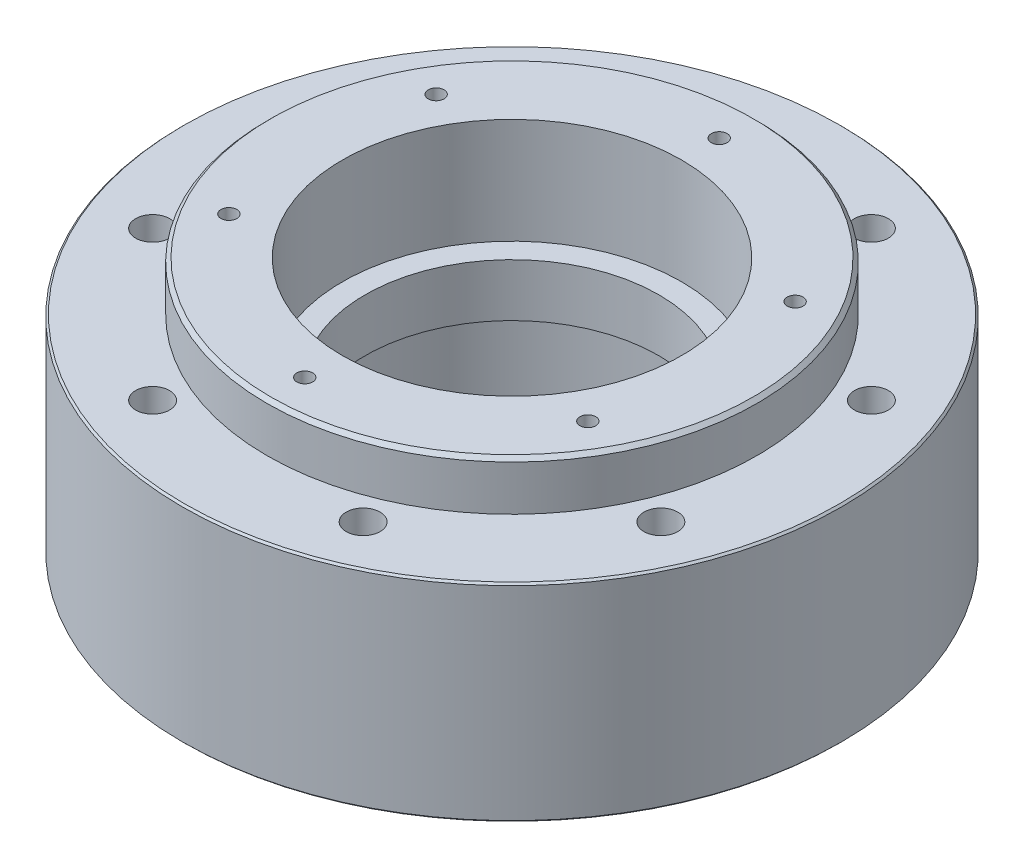
SolidWorks part; units mm, degrees
material "普通碳钢"
ref_plane "Front Plane" through (0, 0, 0) normal (0, 0, 1) x (1, 0, 0)
ref_plane "Top Plane" through (0, 0, 0) normal (0, 1, 0) x (1, 0, 0)
ref_plane "Right Plane" through (0, 0, 0) normal (1, 0, 0) x (0, 0, -1)
sketch "Sketch1" plane through (0, 0, 0) normal (0, 1, 0) x (1, 0, 0)
  circle A0 centre (0, 0) radius 87.5
  dimension "D1" = 175
extrude "Boss-Extrude1" add sketch "Sketch1" along normal blind 55
sketch "Sketch2" plane through (0, 55, 0) normal (0, 1, 0) x (1, 0, 0)
  circle A0 centre (0, 0) radius 65
  dimension "D1" = 130
extrude "Boss-Extrude2" add sketch "Sketch2" along normal blind 13
sketch "Sketch3" plane through (0, 0, 0) normal (0, -1, 0) x (1, 0, 0)
  circle A0 centre (0, 0) radius 57.5
  dimension "D1" = 115
extrude "Boss-Extrude3" add sketch "Sketch3" along normal blind 5
sketch "Sketch4" plane through (0, -5, 0) normal (0, -1, 0) x (1, 0, 0)
  circle A0 centre (0, 0) radius 45
  dimension "D1" = 90
extrude "Cut-Extrude1" cut sketch "Sketch4" against normal blind 31
sketch "Sketch5" plane through (0, 68, 0) normal (0, 1, 0) x (1, 0, 0)
  circle A0 centre (0, 0) radius 45
  dimension "D1" = 90
extrude "Cut-Extrude2" cut sketch "Sketch5" against normal blind 28
sketch "Sketch6" plane through (0, 40, 0) normal (0, 1, 0) x (1, 0, 0)
  circle A0 centre (0, 0) radius 39
  dimension "D1" = 78
extrude "Cut-Extrude3" cut sketch "Sketch6" against normal through all
chamfer "Chamfer1" distance 1 angle 45 2 edges at (0, 68, 65) (0, -5, -57.5)
hole_wizard "Hole size (% based on socket head cap screw type)1" positions "Sketch8" profile "Sketch7" counterbore size "M8" standard "GB" end condition through all
sketch "Sketch8" plane through (0, 0, 0) normal (0, -1, 0) x (-1, 0, 0)
  line L0 (0, 0) -> (0, 104.7926) construction
  line L2 (0, 0) -> (-67.4432, 27.9359) construction
  point P13 (-67.4432, 27.9359)
  dimension "D3" = 67.5
  dimension "D4" = 73
sketch "Sketch7" plane through (67.4432, 0, -27.9359) normal (1, 0, 0) x (0, 0, -1)
  line L0 (0, 0) -> (0, 68)
  line L1 (0, 68) -> (4.5, 68)
  line L3 (4.5, 68) -> (4.5, 30)
  line L4 (4.5, 30) -> (7.5, 30)
  line L5 (7.5, 30) -> (7.5, 0)
  line L7 (7.5, 0) -> (0, 0)
  line L11 (0, -6.35) -> (0, 107.95) construction
  dimension "通孔孔直径" = 9
  dimension "通孔孔深度" = 68
  dimension "柱形沉头孔直径" = 15
  dimension "柱形沉头孔深度" = 30
pattern_circular "CirPattern1" count 8 over 360 about axis through (0, 0, 0) along (0, 1, 0) of "Hole size (% based on socket head cap screw type)1"
chamfer "Chamfer2" distance 0.5 angle 45 2 edges at (0, 55, 87.5) (0, 0, 87.5)
sketch "Sketch12" plane through (0, 68, 0) normal (0, 1, 0) x (1, 0, 0)
  circle A0 centre (0, -50) radius 2.5
  circle A1 centre (0, 0) radius 39 construction
  dimension "D2" = 0
  dimension "D3" = 5
  dimension "D1" = 50
extrude "Cut-Extrude7" cut sketch "Sketch12" against normal blind 22.5
cosmetic thread "Cosmetic Thread2" [suppressed] parameters "D1"=10, "D2"=6
hole_wizard "M10 Tapped Hole1" positions "Sketch14" profile "Sketch13" tap size "M10" standard "GB"
sketch "Sketch14" plane through (0, 0, 0) normal (0, -1, 0) x (-1, 0, 0)
  line L0 (0, 0) -> (106.9821, 0) construction
  line L2 (0, 0) -> (0, 67.5) construction
  point P0 (0, 67.5)
  dimension "D1" = 90
  dimension "D2" = 67.5
sketch "Sketch13" plane through (0, 0, -67.5) normal (1, 0, 0) x (0, 0, -1)
  line L0 (0, 0) -> (0, 40.0537)
  line L1 (0, 40.0537) -> (4.25, 37.5)
  line L2 (4.25, 37.5) -> (4.25, 0)
  line L5 (4.25, 0) -> (0, 0)
  line L10 (0, 40.0537) -> (-4.25, 37.5) construction
  line L11 (0, -6.35) -> (0, 107.95) construction
  dimension "螺纹孔钻头直径" = 8.5
  dimension "螺纹孔钻头深度" = 37.5
  dimension "导头角度" = 118
cosmetic thread "Cosmetic thread 3" parameters "D1"=30, "D2"=10
pattern_circular "CirPattern2" count 8 over 360 about axis through (0, 0, 0) along (0, 1, 0) of "M10 Tapped Hole1"
hole_wizard "M5 Tapped Hole1" positions "Sketch16" profile "Sketch15" tap size "M5" standard "GB"
sketch "Sketch16" plane through (0, 68, 0) normal (0, 1, 0) x (1, 0, 0)
  line L0 (0, 0) -> (0, -64.2731) construction
  line L2 (0, 0) -> (0, -55) construction
  point P0 (0, -55)
  dimension "D1" = 55
  dimension "D2" = 0
sketch "Sketch15" plane through (0, 68, 55) normal (1, 0, 0) x (0, 0, 1)
  line L0 (0, 0) -> (0, 15.2618)
  line L1 (0, 15.2618) -> (2.1, 14)
  line L2 (2.1, 14) -> (2.1, 0)
  line L5 (2.1, 0) -> (0, 0)
  line L10 (0, 15.2618) -> (-2.1, 14) construction
  line L11 (0, -6.35) -> (0, 107.95) construction
  dimension "螺纹孔钻头直径" = 4.2
  dimension "螺纹孔钻头深度" = 14
  dimension "导头角度" = 118
cosmetic thread "Cosmetic thread 2" parameters "D1"=10, "D2"=5
pattern_circular "CirPattern3" count 6 over 360 about axis through (0, 0, 0) along (0, 1, 0) of "M5 Tapped Hole1"
